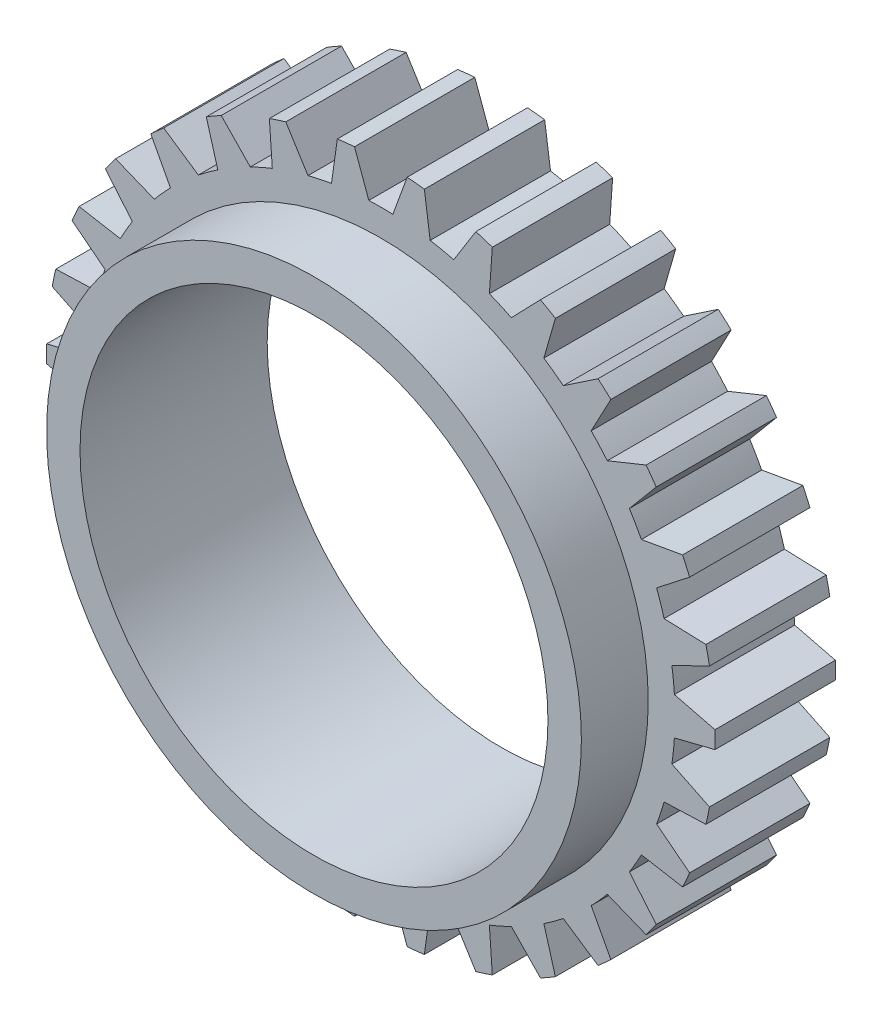
from build123d import *

# Parameters (mm, degrees)
CUT_EXTRUDE1_START = -10
CUT_EXTRUDE1_DEPTH = 10
CIRPATTERN1_COUNT  = 30


with BuildPart() as part:
    # Sketch1 → Revolve1 (revolve)
    with BuildSketch(Plane(origin=(0, 0, 0), x_dir=(0, 0, -1), z_dir=(1, 0, 0)), mode=Mode.PRIVATE) as revolve1_sk:
        Polygon((0, 17.5), (0, 20), (5, 20), (5, 25), (14, 25), (14, 17.5), align=None)
    revolve(revolve1_sk.sketch.rotate(Axis((0, 0, 22.600622446), (0, 0, -1)), 90), axis=Axis((0, 0, 22.600622446), (0, 0, -1)))

    # Sketch2 → Cut-Extrude1 (cut)
    with BuildSketch(Plane.XY.offset(-5).offset(CUT_EXTRUDE1_START)):
        with BuildLine():
            Line((-0.9, -21.9815832), (-1.970310308, -24.922236603))
            ThreePointArc((-1.970310308, -24.922236603), (-0.985922139, -24.980551586), (0, -25))
            Line((0, -25), (0, -22))
            ThreePointArc((0, -22), (-0.450094206, -21.995395318), (-0.9, -21.9815832))
        make_face()
        with BuildLine():
            ThreePointArc((0.9, -21.9815832), (0.450094206, -21.995395318), (0, -22))
            Line((0, -22), (0, -25))
            ThreePointArc((0, -25), (0.985922139, -24.980551586), (1.970310308, -24.922236603))
            Line((1.970310308, -24.922236603), (0.9, -21.9815832))
        make_face()
    cut_extrude1 = extrude(amount=CUT_EXTRUDE1_DEPTH, mode=Mode.SUBTRACT)

    # CirPattern1: Cut-Extrude1 ×30 about axis
    cirpattern1_axis = Axis((0, 0, 0), (0, 0, 1))
    for i in range(1, CIRPATTERN1_COUNT):
        add(cut_extrude1.rotate(cirpattern1_axis, i * 360 / CIRPATTERN1_COUNT), mode=Mode.SUBTRACT)


solid = part.part
